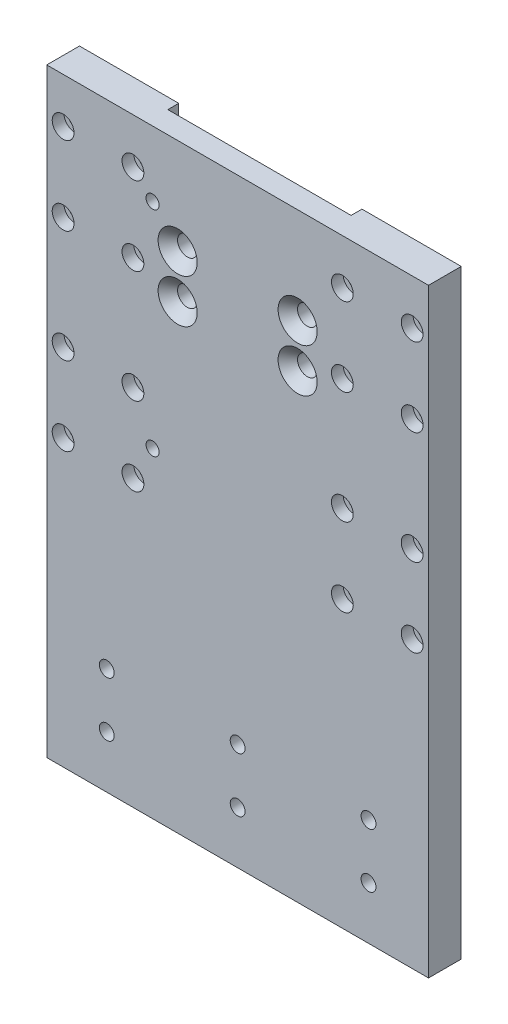
from build123d import *

# Parameters (mm, degrees)
SKETCH_1_W                   = 175
SKETCH_1_H                   = 275
EXTRUDE_1_DEPTH              = 10
SKETCH_10_W                  = 45.5
SKETCH_10_H                  = 275
EXTRUDE_2_DEPTH              = 5
HOLE_WIZARD_M8_1_D           = 9
HOLE_WIZARD_M8_1_CSINK_D     = 17.92
HOLE_WIZARD_M8_1_CSINK_ANGLE = 90
HOLE_WIZARD_M8_1_2_D         = 6.8
HOLE_WIZARD_M5_1_D           = 5.5
HOLE_WIZARD_M5_1_CBORE_D     = 10
HOLE_WIZARD_M5_1_CBORE_DEPTH = 5.4
F_6_0MM_1_D                  = 6


with BuildPart() as part:
    # 草图1 → 凸台-拉伸1 (new body)
    with BuildSketch(Plane.XY):
        Rectangle(SKETCH_1_W, SKETCH_1_H)
    extrude(amount=EXTRUDE_1_DEPTH)

    # 草图10 → 凸台-拉伸2 (add)
    with BuildSketch(Plane(origin=(0, 0, 0), x_dir=(-1, 0, 0), z_dir=(0, 0, -1))):
        with Locations((-64.75, 0)):
            Rectangle(SKETCH_10_W, SKETCH_10_H)
        with Locations((64.75, 0)):
            Rectangle(SKETCH_10_W, SKETCH_10_H)
    extrude(amount=EXTRUDE_2_DEPTH)

    # Hole Wizard M8 _1 (through all)
    with Locations(Plane.XY.offset(10)):
        with Locations((-27.5, 93.5), (-27.5, 73.5), (27.5, 93.5), (27.5, 73.5)):
            CounterSinkHole(HOLE_WIZARD_M8_1_D / 2, HOLE_WIZARD_M8_1_CSINK_D / 2, counter_sink_angle=HOLE_WIZARD_M8_1_CSINK_ANGLE)

    # Hole Wizard M8 _1 2 (through all)
    with Locations(Plane.XY.offset(10)):
        with Locations((0, -113.5), (-60, -113.5), (60, -113.5), (0, -88.5), (-60, -88.5), (60, -88.5)):
            Hole(HOLE_WIZARD_M8_1_2_D / 2)

    # M5 六角凹头螺钉的柱形沉头孔1 (through all)
    with Locations(Plane.XY.offset(10)):
        with Locations((-80, 116.75), (-48, 116.75), (-80, 80.75), (-48, 80.75), (-80, 29.25), (-48, 29.25), (-80, -6.75), (-48, -6.75), (48, -6.75), (80, -6.75), (48, 29.25), (80, 29.25), (48, 80.75), (80, 80.75), (48, 116.75), (80, 116.75)):
            CounterBoreHole(HOLE_WIZARD_M5_1_D / 2, HOLE_WIZARD_M5_1_CBORE_D / 2, HOLE_WIZARD_M5_1_CBORE_DEPTH)

    # Ø6.0mm 暗销孔1 (through all)
    with Locations(Plane.XY.offset(10)):
        with Locations((-39, 107.5), (-39, 9.5)):
            Hole(F_6_0MM_1_D / 2)


solid = part.part
